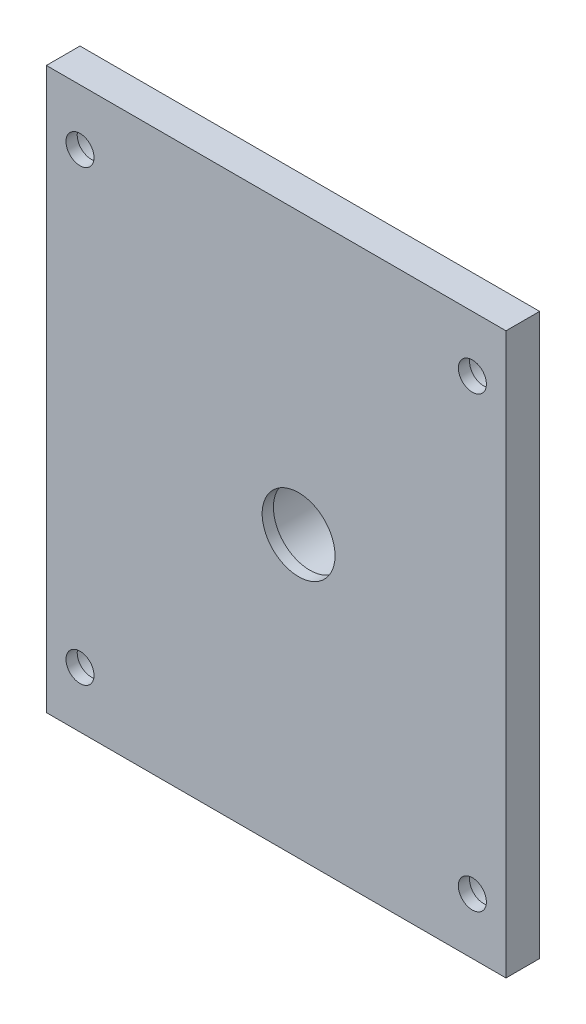
from build123d import *

# Parameters (mm, degrees)
SKETCH_1_W           = 82
SKETCH_1_H           = 100
EXTRUDE_1_DEPTH      = 6
SKETCH_3_R           = 12
EXTRUDE_3_DEPTH      = 14
SKETCH_7_R           = 4
CUT_EXTRUDE_4_DEPTH  = 4
SKETCH_5_R           = 6.5
CUT_EXTRUDE_8_DEPTH  = 2
SKETCH_11_R          = 7.5
CUT_EXTRUDE_9_DEPTH  = 12
SKETCH_12_R          = 2.5
CUT_EXTRUDE_10_DEPTH = 6


with BuildPart() as part:
    # 草图1 → 凸台-拉伸1 (new body)
    with BuildSketch(Plane.XY):
        Rectangle(SKETCH_1_W, SKETCH_1_H)
    extrude(amount=EXTRUDE_1_DEPTH)

    # 草图3 → 凸台-拉伸3 (add)
    with BuildSketch(Plane.XY.offset(6)):
        with Locations((4, 0)):
            Circle(SKETCH_3_R)
    extrude(amount=-EXTRUDE_3_DEPTH)

    # 草图7 → 切除-拉伸4 (cut)
    with BuildSketch(Plane(origin=(0, 0, 0), x_dir=(-1, 0, 0), z_dir=(0, 0, -1))):
        with Locations((-35, 40)):
            Circle(SKETCH_7_R)
        with Locations(Location((-35, -40, 0), (0, 0, 180))):
            Circle(SKETCH_7_R)
        with Locations((35, -40)):
            Circle(SKETCH_7_R)
        with Locations(Location((35, 40, 0), (0, 0, 180))):
            Circle(SKETCH_7_R)
    extrude(amount=-CUT_EXTRUDE_4_DEPTH, mode=Mode.SUBTRACT)

    # 草图5 → 切除-拉伸8 (cut)
    with BuildSketch(Plane.XY.offset(6)):
        with Locations((4, 0)):
            Circle(SKETCH_5_R)
    extrude(amount=-CUT_EXTRUDE_8_DEPTH, mode=Mode.SUBTRACT)

    # 草图11 → 切除-拉伸9 (cut)
    with BuildSketch(Plane(origin=(0, 0, -8), x_dir=(-1, 0, 0), z_dir=(0, 0, -1))):
        with Locations((-4, 0)):
            Circle(SKETCH_11_R)
    extrude(amount=-CUT_EXTRUDE_9_DEPTH, mode=Mode.SUBTRACT)

    # 草图12 → 切除-拉伸10 (cut)
    with BuildSketch(Plane(origin=(0, 0, 0), x_dir=(-1, 0, 0), z_dir=(0, 0, -1))):
        with Locations((-35, -40)):
            Circle(SKETCH_12_R)
        with Locations((-35, 40)):
            Circle(SKETCH_12_R)
        with Locations((35, -40)):
            Circle(SKETCH_12_R)
        with Locations((35, 40)):
            Circle(SKETCH_12_R)
    extrude(amount=-CUT_EXTRUDE_10_DEPTH, mode=Mode.SUBTRACT)


solid = part.part
